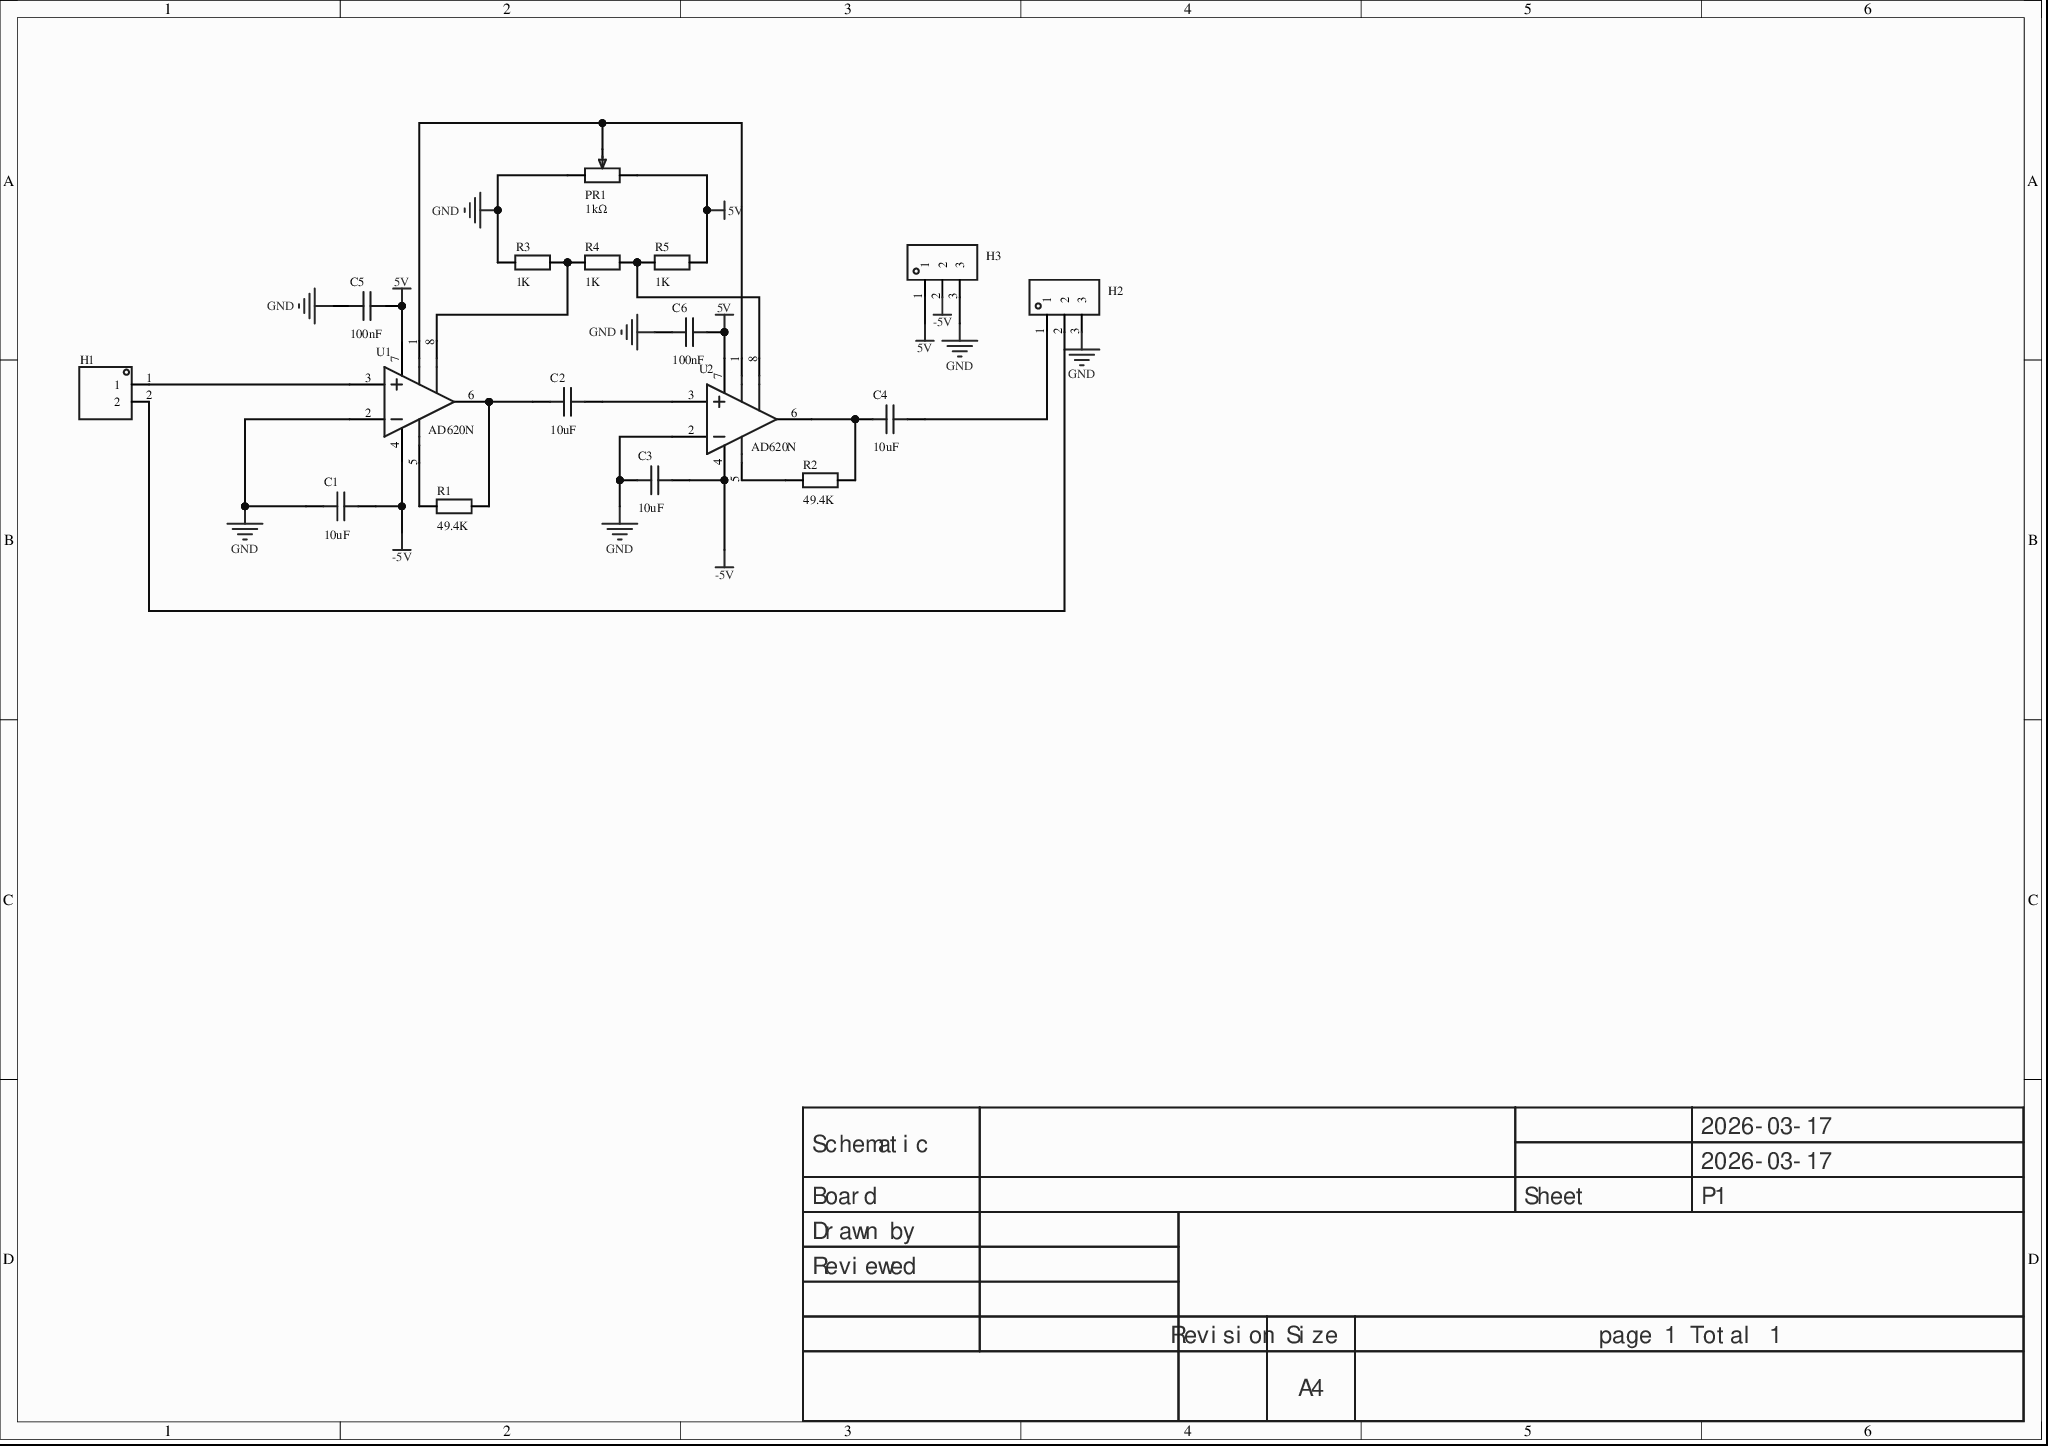
[diagram p0: MISC89042-3.schdoc]
# Altium project MISC89042-2.PrjPcb
1 sheet, 17 parts. Net scope: global (net labels, ports and power ports of the same name join across sheets).
Board file: MISC89042.pcbdoc

## Sheet MISC89042-3.schdoc
size 297 x 209 mm; Version: V1.0; @Project Name: MISC89042; @Update Date: 2026-03-17; @Create Date: 2026-03-17; @Board Name: MISC89042; @Create Time: 14:54:38; @Page Count: 1; @Page No: 1; @Schematic Name: MISC89042; @Update Time: 14:54:38; Size: A4

### Parts
C1  10uF  [C0603]
C2  10uF  [C0603]
C3  10uF  [C0603]
C4  10uF  [C0603]
C5  100nF  [C0603]
C6  100nF  [C0603]
H1  (no value)  [HDR-TH_2P-P2.54-V-M-1]
H2  (no value)  [HDR-TH_3P-P2.54-V-M]
H3  (no value)  [HDR-TH_3P-P2.54-V-M]
PR1  1kΩ  [R_3296]
R1  49.4K  [R0603]
R2  49.4K  [R0603]
R3  1K  [R0603]
R4  1K  [R0603]
R5  1K  [R0603]
U1  AD620N  [SOIC-8_L5.0-W4.0-P1.27-LS6.0-BL]
U2  AD620N  [SOIC-8_L5.0-W4.0-P1.27-LS6.0-BL]

### Nets
5V: C5.2 C6.2 H3.1 PR1.1 R5.2 U1.7(V+) U2.7(V+)
-5V: C1.2 C3.2 H3.2 U1.4(V-) U2.4(V-)
GND: C1.1 C3.1 C5.1 C6.1 H2.3 H3.3 PR1.3 R3.1 U1.2(IN+) U2.2(IN+)
NetC2_1: C2.1 R1.2 U1.6(OUT)
NetC2_2: C2.2 U2.3(IN-)
NetC4_1: C4.1 R2.2 U2.6(OUT)
NetC4_2: C4.2 H2.1
NetH1_1: H1.1 U1.3(IN-)
NetH1_2: H1.2 H2.2
NetPR1_2: PR1.2 U1.1(RG) U2.1(RG)
NetR1_1: R1.1 U1.5(REF)
NetR2_1: R2.1 U2.5(REF)
NetR3_2: R3.2 R4.1 U1.8(RG)
NetR4_2: R4.2 R5.1 U2.8(RG)

### Notes on the sheet
- 2026-03-17
- Schematic
- Board
- Sheet
- P1
- Drawn by
- Reviewed
- Revision
- Size
- A4
- page 1 Total 1

### Library data of the parts
C1-C6 = CAP_0603: Symbol: Capacitance; ConvertToPcb: yes; ModelId: ac125912035d415993ca9572d50418b10819f05c4eef4c71ace90d822a990e87; ModelName: C0603_L1.6-W0.8-H0.8; ModelTransform: 62.992,31.496,0,0,0,0,0,0,0; Device: CAP_0603; AddInBom: yes; Supplier Footprint: 0603; FootprintName: C0603
  C1-C4: Value: 10uF
  C5 C6: Value: 100nF
H1 = HDR-M_2.54_1x2P: Symbol: 210S-1*2P L=11.6MMGold-plated black; ConvertToPcb: yes; ModelId: 79b2e9f2d70a4d68a1b7098f27c6d4c50819f05c4eef4c71ace90d822a990e87; ModelName: HDR-M-2.54_1x2; ModelTransform: 200,100,0,0,0,0,0,0,-118.11; Device: HDR-M_2.54_1x2P; AddInBom: yes; SupplierPart: C124375; Supplier Footprint: 插件; FootprintName: HDR-TH_2P-P2.54-V-M-1
H2 H3 = HDR-M_2.54_1x3P: AddInBom: yes; ModelId: bb473b6d38ff42a99216a4fcdbdcc4cb0819f05c4eef4c71ace90d822a990e87; ModelName: HDR-TH_3P-P2.54-M-LI-1X3P; ModelTransform: 300.03877,100,0,0,0,0,0,0,-118.11; Symbol: HDR-M_2.54_1x3P; Device: HDR-M_2.54_1x3P; ConvertToPcb: yes; FootprintName: HDR-TH_3P-P2.54-V-M; SupplierPart: C2937625; Supplier Footprint: 插件
PR1 = R_3296: ConvertToPcb: yes; ModelId: b182808559bb43bda9e7de64b64134cb0819f05c4eef4c71ace90d822a990e87; ModelName: 3296W; ModelTransform: 373.98,188.96,590.49,180,0,0,0,0,-140; Symbol: R_3296; Device: R_3296; Value: 1kΩ; AddInBom: yes; Supplier Footprint: 直插; FootprintName: R_3296
R1-R5 = Res_0603: Symbol: Resistor; ConvertToPcb: yes; ModelId: fc143cca1e79419f9cd78b61e9279f080819f05c4eef4c71ace90d822a990e87; ModelTransform: 31.8897,63.7794,0,90,0,0,0,0,0; Device: Res_0603; AddInBom: yes; Supplier Footprint: 0603; FootprintName: R0603; ModelName: R0603
  R1 R2: Value: 49.4K
  R3-R5: Value: 1K
U1 U2 = AD620BRZ-RL-JSM: Low-drift, low-power instrumentation amplifier, gain setting range 1 to 10000; Manufacturer: JSMSEMI(杰盛微); Relevance: []; AddInBom: yes; ModelId: 7abc64c95a1a4a04a4ef38f9097c870b0819f05c4eef4c71ace90d822a990e87; ModelTransform: 192.913,236.22,0,0,0,0,0,0,0; Symbol: AD620BRZ-RL-JSM; Device: AD620BRZ-RL-JSM; Manufacturer Part: AD620N; LCSC Part Name: AD620BRZ-RL-JSM; SupplierPart: C49369931; Supplier Footprint: SOP-8; JLCPCB Part Class: Extended Part; Datasheet: https://item.szlcsc.com/datasheet/AD620BRZ-RL-JSM/51877593.html; Supplier: LCSC; ConvertToPcb: yes; FootprintName: SOIC-8_L5.0-W4.0-P1.27-LS6.0-BL; ModelName: SOIC-8_L5.0-W4.0-P1.27-LS6.0-BL